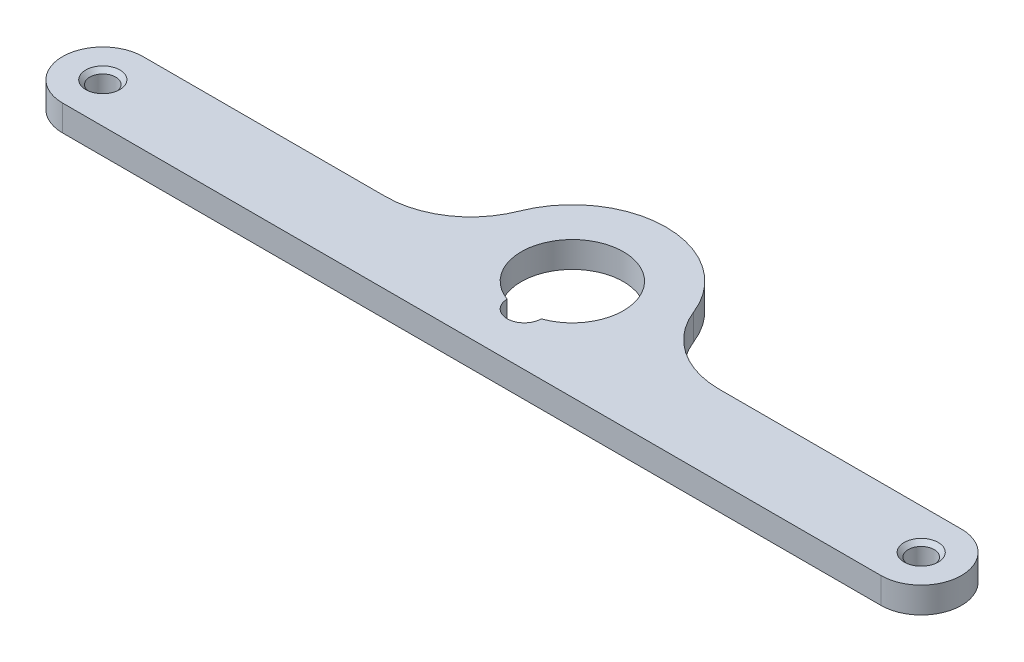
from build123d import *

# Parameters (mm, degrees)
SKETCH1_R           = 2.413
BOSS_EXTRUDE1_DEPTH = 2.413
CHAMFER1_SIZE       = 0.762


with BuildPart() as part:
    # Sketch1 → Boss-Extrude1 (new, symmetric)
    with BuildSketch(Plane(origin=(0, 0, 0), x_dir=(1, 0, 0), z_dir=(0, 1, 0))):
        with BuildLine():
            Line((-76.2, -18.7325), (76.2, -18.7325))
            ThreePointArc((76.2, -18.7325), (83.693, -11.2395), (76.2, -3.7465))
            Line((76.2, -3.7465), (31.039358608, -3.7465))
            ThreePointArc((31.039358608, -3.7465), (22.086845014, -0.981348411), (16.253078783, 6.35082279))
            ThreePointArc((16.253078783, 6.35082279), (0, 17.4498), (-16.253078783, 6.35082279))
            ThreePointArc((-16.253078783, 6.35082279), (-22.086845014, -0.981348411), (-31.039358608, -3.7465))
            Line((-31.039358608, -3.7465), (-76.2, -3.7465))
            ThreePointArc((-76.2, -3.7465), (-83.693, -11.2395), (-76.2, -18.7325))
        make_face()
        with Locations(Location((76.2, -11.2395, 0), (0, 0, 270))):
            Circle(SKETCH1_R, mode=Mode.SUBTRACT)
        with Locations(Location((-76.2, -11.2395, 0), (0, 0, 270))):
            Circle(SKETCH1_R, mode=Mode.SUBTRACT)
        with BuildLine():
            ThreePointArc((3.174972166, -8.966794468), (0, 9.5123), (-3.174972166, -8.966794468))
            ThreePointArc((-3.174972166, -8.966794468), (0, -12.1285), (3.174972166, -8.966794468))
        make_face(mode=Mode.SUBTRACT)
    extrude(amount=BOSS_EXTRUDE1_DEPTH, both=True)

    # Chamfer1
    chamfer1_edges = [part.edges().sort_by_distance(p)[0] for p in [
        (76.2, -2.413, 8.8265),
        (76.2, 2.413, 8.8265),
        (-76.2, -2.413, 8.8265),
        (-76.2, 2.413, 8.8265),
    ]]
    chamfer(chamfer1_edges, length=CHAMFER1_SIZE)


solid = part.part
